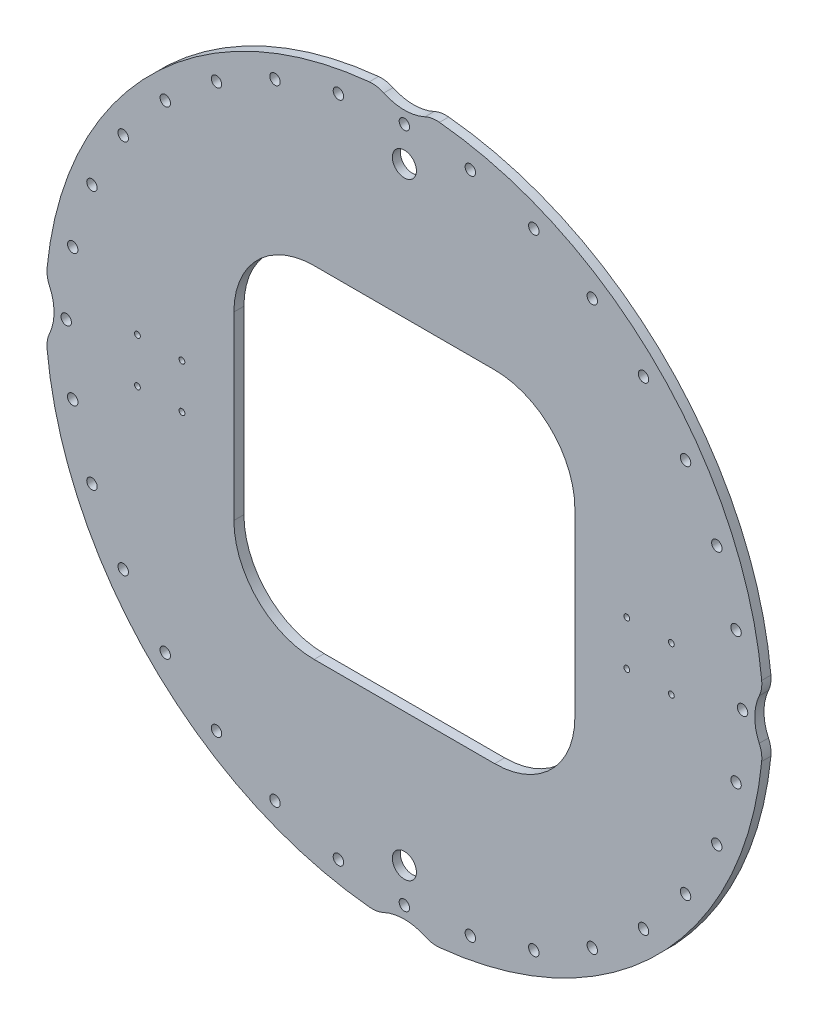
from build123d import *

# Parameters (mm, degrees)
SKETCH1_R           = 13
SKETCH1_R_2         = 30
SKETCH1_R_3         = 7.25
BOSS_EXTRUDE1_DEPTH = 25
SKETCH2_R           = 870
SKETCH2_R_2         = 675
CUT_EXTRUDE1_DEPTH  = 5
SKETCH3_R           = 1126.547936792
SKETCH3_R_2         = 762.256112449
CUT_EXTRUDE2_DEPTH  = 2


with BuildPart() as part:
    # Sketch1 → Boss-Extrude1 (new body)
    with BuildSketch(Plane.XY):
        with BuildLine():
            ThreePointArc((-87.472233281, 890.715222956), (-632.860569162, 632.860569162), (-890.715222956, 87.472233281))
            ThreePointArc((-890.715222956, 87.472233281), (-890.074747514, 68.984719363), (-884.613856025, 51.310527902))
            ThreePointArc((-884.613856025, 51.310527902), (-873.35, 0), (-884.613856025, -51.310527902))
            ThreePointArc((-884.613856025, -51.310527902), (-890.074747514, -68.984719363), (-890.715222956, -87.472233281))
            ThreePointArc((-890.715222956, -87.472233281), (-632.860569162, -632.860569162), (-87.472233281, -890.715222956))
            ThreePointArc((-87.472233281, -890.715222956), (-68.984719363, -890.074747514), (-51.310527902, -884.613856025))
            ThreePointArc((-51.310527902, -884.613856025), (0, -873.35), (51.310527902, -884.613856025))
            ThreePointArc((51.310527902, -884.613856025), (68.984719363, -890.074747514), (87.472233281, -890.715222956))
            ThreePointArc((87.472233281, -890.715222956), (632.860569162, -632.860569162), (890.715222956, -87.472233281))
            ThreePointArc((890.715222956, -87.472233281), (890.074747514, -68.984719363), (884.613856025, -51.310527902))
            ThreePointArc((884.613856025, -51.310527902), (873.35, 0), (884.613856025, 51.310527902))
            ThreePointArc((884.613856025, 51.310527902), (890.074747514, 68.984719363), (890.715222956, 87.472233281))
            ThreePointArc((890.715222956, 87.472233281), (632.860569162, 632.860569162), (87.472233281, 890.715222956))
            ThreePointArc((87.472233281, 890.715222956), (68.984719363, 890.074747514), (51.310527902, 884.613856025))
            ThreePointArc((51.310527902, 884.613856025), (0, 873.35), (-51.310527902, 884.613856025))
            ThreePointArc((-51.310527902, 884.613856025), (-68.984719363, 890.074747514), (-87.472233281, 890.715222956))
        make_face()
        with Locations((0, 843)):
            Circle(SKETCH1_R, mode=Mode.SUBTRACT)
        with Locations((0, 757)):
            Circle(SKETCH1_R_2, mode=Mode.SUBTRACT)
        with Locations((554.5, 55.5)):
            Circle(SKETCH1_R_3, mode=Mode.SUBTRACT)
        with Locations((665.5, 55.5)):
            Circle(SKETCH1_R_3, mode=Mode.SUBTRACT)
        with Locations((665.5, -55.5)):
            Circle(SKETCH1_R_3, mode=Mode.SUBTRACT)
        with Locations((554.5, -55.5)):
            Circle(SKETCH1_R_3, mode=Mode.SUBTRACT)
        with Locations(Location((0, -757, 0), (0, 0, 180))):
            Circle(SKETCH1_R_2, mode=Mode.SUBTRACT)
        with Locations(Location((-665.5, -55.5, 0), (0, 0, 180))):
            Circle(SKETCH1_R_3, mode=Mode.SUBTRACT)
        with Locations(Location((-554.5, -55.5, 0), (0, 0, 180))):
            Circle(SKETCH1_R_3, mode=Mode.SUBTRACT)
        with Locations(Location((-665.5, 55.5, 0), (0, 0, 180))):
            Circle(SKETCH1_R_3, mode=Mode.SUBTRACT)
        with Locations(Location((-554.5, 55.5, 0), (0, 0, 180))):
            Circle(SKETCH1_R_3, mode=Mode.SUBTRACT)
        with Locations((164.46114146, 826.80199138)):
            Circle(SKETCH1_R, mode=Mode.SUBTRACT)
        with Locations((322.602133484, 778.830445907)):
            Circle(SKETCH1_R, mode=Mode.SUBTRACT)
        with Locations((468.345706436, 700.928883171)):
            Circle(SKETCH1_R, mode=Mode.SUBTRACT)
        with Locations((596.09101654, 596.09101654)):
            Circle(SKETCH1_R, mode=Mode.SUBTRACT)
        with Locations((700.928883171, 468.345706436)):
            Circle(SKETCH1_R, mode=Mode.SUBTRACT)
        with Locations((778.830445907, 322.602133484)):
            Circle(SKETCH1_R, mode=Mode.SUBTRACT)
        with Locations((826.80199138, 164.46114146)):
            Circle(SKETCH1_R, mode=Mode.SUBTRACT)
        with Locations((843, 0)):
            Circle(SKETCH1_R, mode=Mode.SUBTRACT)
        with Locations((826.80199138, -164.46114146)):
            Circle(SKETCH1_R, mode=Mode.SUBTRACT)
        with Locations((778.830445907, -322.602133484)):
            Circle(SKETCH1_R, mode=Mode.SUBTRACT)
        with Locations((700.928883171, -468.345706436)):
            Circle(SKETCH1_R, mode=Mode.SUBTRACT)
        with Locations((596.09101654, -596.09101654)):
            Circle(SKETCH1_R, mode=Mode.SUBTRACT)
        with Locations((468.345706436, -700.928883171)):
            Circle(SKETCH1_R, mode=Mode.SUBTRACT)
        with Locations((322.602133484, -778.830445907)):
            Circle(SKETCH1_R, mode=Mode.SUBTRACT)
        with Locations((164.46114146, -826.80199138)):
            Circle(SKETCH1_R, mode=Mode.SUBTRACT)
        with Locations((0, -843)):
            Circle(SKETCH1_R, mode=Mode.SUBTRACT)
        with Locations((-164.46114146, -826.80199138)):
            Circle(SKETCH1_R, mode=Mode.SUBTRACT)
        with Locations((-322.602133484, -778.830445907)):
            Circle(SKETCH1_R, mode=Mode.SUBTRACT)
        with Locations((-468.345706436, -700.928883171)):
            Circle(SKETCH1_R, mode=Mode.SUBTRACT)
        with Locations((-596.09101654, -596.09101654)):
            Circle(SKETCH1_R, mode=Mode.SUBTRACT)
        with Locations((-700.928883171, -468.345706436)):
            Circle(SKETCH1_R, mode=Mode.SUBTRACT)
        with Locations((-778.830445907, -322.602133484)):
            Circle(SKETCH1_R, mode=Mode.SUBTRACT)
        with Locations((-826.80199138, -164.46114146)):
            Circle(SKETCH1_R, mode=Mode.SUBTRACT)
        with Locations((-843, 0)):
            Circle(SKETCH1_R, mode=Mode.SUBTRACT)
        with Locations((-826.80199138, 164.46114146)):
            Circle(SKETCH1_R, mode=Mode.SUBTRACT)
        with Locations((-778.830445907, 322.602133484)):
            Circle(SKETCH1_R, mode=Mode.SUBTRACT)
        with Locations((-700.928883171, 468.345706436)):
            Circle(SKETCH1_R, mode=Mode.SUBTRACT)
        with Locations((-596.09101654, 596.09101654)):
            Circle(SKETCH1_R, mode=Mode.SUBTRACT)
        with Locations((-468.345706436, 700.928883171)):
            Circle(SKETCH1_R, mode=Mode.SUBTRACT)
        with Locations((-322.602133484, 778.830445907)):
            Circle(SKETCH1_R, mode=Mode.SUBTRACT)
        with Locations((-164.46114146, 826.80199138)):
            Circle(SKETCH1_R, mode=Mode.SUBTRACT)
        with BuildLine():
            Line((-225, -425), (225, -425))
            ThreePointArc((225, -425), (366.421356237, -366.421356237), (425, -225))
            Line((425, -225), (425, 225))
            ThreePointArc((425, 225), (366.421356237, 366.421356237), (225, 425))
            Line((225, 425), (-225, 425))
            ThreePointArc((-225, 425), (-366.421356237, 366.421356237), (-425, 225))
            Line((-425, 225), (-425, -225))
            ThreePointArc((-425, -225), (-366.421356237, -366.421356237), (-225, -425))
        make_face(mode=Mode.SUBTRACT)
    extrude(amount=BOSS_EXTRUDE1_DEPTH)

    # Sketch2 → Cut-Extrude1 (cut)
    with BuildSketch(Plane(origin=(0, 0, 0), x_dir=(-1, 0, 0), z_dir=(0, 0, -1))):
        Circle(SKETCH2_R)
        Circle(SKETCH2_R_2, mode=Mode.SUBTRACT)
    extrude(amount=-CUT_EXTRUDE1_DEPTH, mode=Mode.SUBTRACT)

    # Sketch3 → Cut-Extrude2 (cut)
    with BuildSketch(Plane(origin=(0, 0, 0), x_dir=(-1, 0, 0), z_dir=(0, 0, -1))):
        Circle(SKETCH3_R)
        Circle(SKETCH3_R_2, mode=Mode.SUBTRACT)
    extrude(amount=-CUT_EXTRUDE2_DEPTH, mode=Mode.SUBTRACT)


solid = part.part
